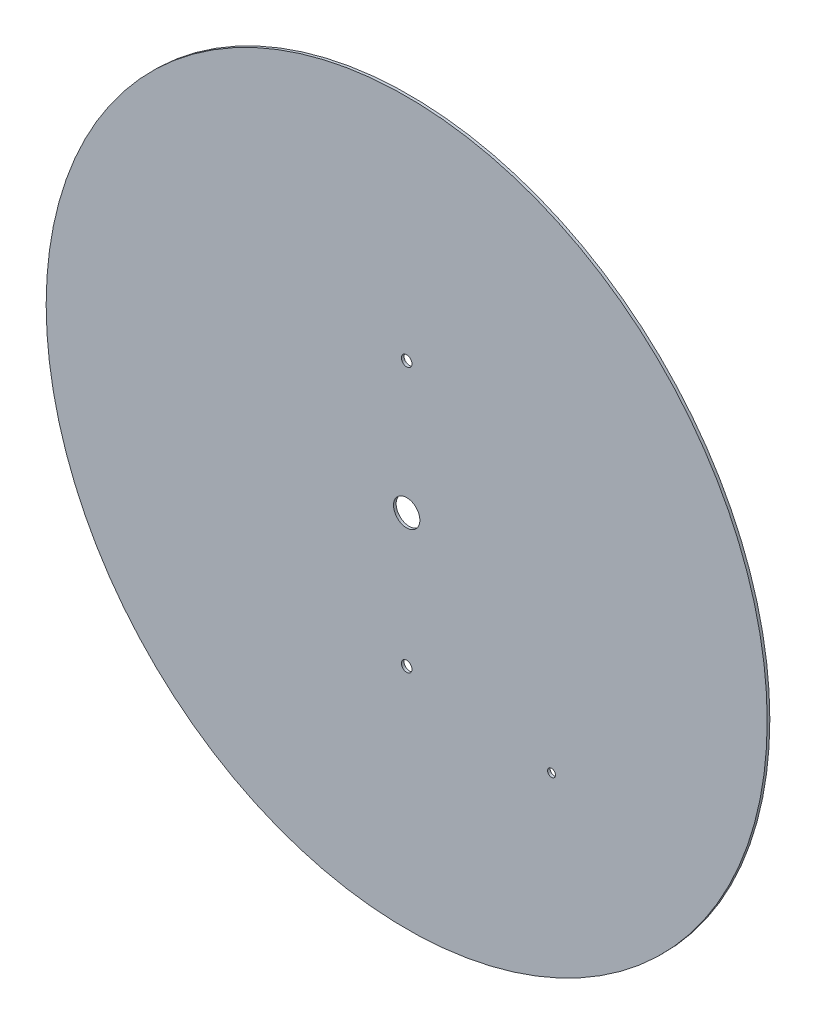
from build123d import *

# Parameters (mm, degrees)
SKETCH_1_R               = 68.5
BOSS_EXTRUDE_1_DEPTH     = 0.5
CUT_EXTRUDE_1_REACH      = 98.875
SKETCH_2_R               = 2.5
CUT_EXTRUDE_2_REACH      = 98.875
SKETCH_3_R               = 1
CUT_EXTRUDE_3_REACH      = 98.875
SKETCH_4_R               = 0.75
BOSS_EXTRUDE_2_DEPTH     = 0.5
CIRCULAR_PATTERN_1_COUNT = 9
CIRCULAR_PATTERN_1_ANGLE = 270
BOSS_EXTRUDE_3_DEPTH     = 0.5
CIRCULAR_PATTERN_2_COUNT = 79
CIRCULAR_PATTERN_2_ANGLE = 263.25
CUT_EXTRUDE_4_REACH      = 98.875
SKETCH_7_R               = 1


with BuildPart() as part:
    # Sketch 1 → Boss-Extrude 1 (new body)
    with BuildSketch(Plane.XY):
        Circle(SKETCH_1_R)
    extrude(amount=BOSS_EXTRUDE_1_DEPTH)

    # Sketch 2 → Cut-Extrude 1 (cut, up to next)
    with BuildSketch(Plane(origin=(0, 0, 0), x_dir=(-1, 0, 0), z_dir=(0, 0, -1)), mode=Mode.PRIVATE) as cut_extrude_1_sk1:
        Circle(SKETCH_2_R)
    cut_extrude_1_tool1 = extrude(cut_extrude_1_sk1.sketch, amount=-CUT_EXTRUDE_1_REACH, mode=Mode.PRIVATE) & part.part
    add(cut_extrude_1_tool1.solids().sort_by_distance((0, 0, 0))[0], mode=Mode.SUBTRACT)

    # Sketch 3 → Cut-Extrude 2 (cut, up to next)
    with BuildSketch(Plane(origin=(0, 0, 0), x_dir=(-1, 0, 0), z_dir=(0, 0, -1)), mode=Mode.PRIVATE) as cut_extrude_2_sk1:
        with Locations((0, 25)):
            Circle(SKETCH_3_R)
    cut_extrude_2_tool1 = extrude(cut_extrude_2_sk1.sketch, amount=-CUT_EXTRUDE_2_REACH, mode=Mode.PRIVATE) & part.part
    add(cut_extrude_2_tool1.solids().sort_by_distance((0, 25, 0))[0], mode=Mode.SUBTRACT)

    # Sketch 4 → Cut-Extrude 3 (cut, up to next)
    with BuildSketch(Plane(origin=(0, 0, 0), x_dir=(-1, 0, 0), z_dir=(0, 0, -1)), mode=Mode.PRIVATE) as cut_extrude_3_sk1:
        with Locations((-27.516659321, -29.031594166)):
            Circle(SKETCH_4_R)
    cut_extrude_3_tool1 = extrude(cut_extrude_3_sk1.sketch, amount=-CUT_EXTRUDE_3_REACH, mode=Mode.PRIVATE) & part.part
    add(cut_extrude_3_tool1.solids().sort_by_distance((27.516659, -29.031594, 0))[0], mode=Mode.SUBTRACT)

    # Sketch 5 → Boss-Extrude 2 (add)
    with BuildSketch(Plane(origin=(0, 0, 0), x_dir=(-1, 0, 0), z_dir=(0, 0, -1))):
        Polygon((-42.779960262, -42.072853481), (-32.173358544, -31.466251763), (-31.466251763, -32.173358544), (-42.072853481, -42.779960262), align=None)
    boss_extrude_2 = extrude(amount=BOSS_EXTRUDE_2_DEPTH)

    # Circular pattern 1: Boss-Extrude 2 ×9 about axis
    circular_pattern_1_axis = Axis((0, 0, 0), (0, 0, 1))
    for i in range(1, CIRCULAR_PATTERN_1_COUNT):
        add(boss_extrude_2.rotate(circular_pattern_1_axis, i * CIRCULAR_PATTERN_1_ANGLE / (CIRCULAR_PATTERN_1_COUNT - 1)))

    # Sketch 6 → Boss-Extrude 3 (add)
    with BuildSketch(Plane(origin=(0, 0, 0), x_dir=(-1, 0, 0), z_dir=(0, 0, -1))):
        Polygon((-45.182625831, -39.481392111), (-37.707542562, -32.838867732), (-37.043290124, -33.586376059), (-44.518373393, -40.228900438), align=None)
    boss_extrude_3 = extrude(amount=BOSS_EXTRUDE_3_DEPTH)

    # Circular pattern 2: Boss-Extrude 3 ×79 about axis, 7 skipped
    circular_pattern_2_axis = Axis((0, 0, 0), (0, 0, 1))
    add([boss_extrude_3.rotate(circular_pattern_2_axis, i * CIRCULAR_PATTERN_2_ANGLE / (CIRCULAR_PATTERN_2_COUNT - 1)) for i in range(1, CIRCULAR_PATTERN_2_COUNT) if i not in (9, 19, 29, 39, 49, 59, 69)])

    # Sketch 7 → Cut-Extrude 4 (cut, up to next)
    with BuildSketch(Plane(origin=(0, 0, 0), x_dir=(-1, 0, 0), z_dir=(0, 0, -1)), mode=Mode.PRIVATE) as cut_extrude_4_sk1:
        with Locations((0, -25.26)):
            Circle(SKETCH_7_R)
    cut_extrude_4_tool1 = extrude(cut_extrude_4_sk1.sketch, amount=-CUT_EXTRUDE_4_REACH, mode=Mode.PRIVATE) & part.part
    add(cut_extrude_4_tool1.solids().sort_by_distance((0, -25.26, 0))[0], mode=Mode.SUBTRACT)


solid = part.part
